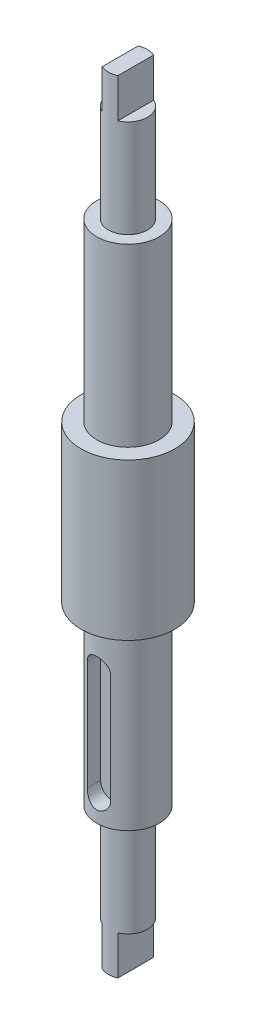
from build123d import *

# Parameters (mm, degrees)
SKETCH1_R           = 6
BOSS_EXTRUDE1_DEPTH = 10
SKETCH2_R           = 4
BOSS_EXTRUDE2_DEPTH = 22.5
SKETCH3_R           = 2.5
BOSS_EXTRUDE3_DEPTH = 12.5
BOSS_EXTRUDE4_START = 22.5
SKETCH4_R           = 4
BOSS_EXTRUDE4_DEPTH = 22.5
BOSS_EXTRUDE5_START = 12.5
SKETCH5_R           = 2.5
BOSS_EXTRUDE5_DEPTH = 12.5
BOSS_EXTRUDE6_START = 5
BOSS_EXTRUDE6_DEPTH = 5
BOSS_EXTRUDE7_DEPTH = 5
CUT_EXTRUDE1_DEPTH  = 2


with BuildPart() as part:
    # Sketch1 → Boss-Extrude1 (new, symmetric)
    with BuildSketch(Plane(origin=(0, 0, 0), x_dir=(1, 0, 0), z_dir=(0, 1, 0))):
        with Locations(Location((0, 0, 0), (0, 0, 270))):
            Circle(SKETCH1_R)
    extrude(amount=BOSS_EXTRUDE1_DEPTH, both=True)

    # Sketch2 → Boss-Extrude2 (add)
    with BuildSketch(Plane(origin=(0, 10, 0), x_dir=(1, 0, 0), z_dir=(0, 1, 0))):
        with Locations(Location((0, 0, 0), (0, 0, 90))):
            Circle(SKETCH2_R)
    extrude(amount=BOSS_EXTRUDE2_DEPTH)

    # Sketch3 → Boss-Extrude3 (add)
    with BuildSketch(Plane(origin=(0, 32.5, 0), x_dir=(1, 0, 0), z_dir=(0, 1, 0))):
        with Locations(Location((0, 0, 0), (0, 0, 270))):
            Circle(SKETCH3_R)
    extrude(amount=BOSS_EXTRUDE3_DEPTH)

    # Sketch4 → Boss-Extrude4 (add)
    with BuildSketch(Plane.XZ.offset(10).offset(BOSS_EXTRUDE4_START)):
        with Locations(Location((0, 0, 0), (0, 0, 270))):
            Circle(SKETCH4_R)
    extrude(amount=-BOSS_EXTRUDE4_DEPTH)

    # Sketch5 → Boss-Extrude5 (add)
    with BuildSketch(Plane.XZ.offset(32.5).offset(BOSS_EXTRUDE5_START)):
        with Locations(Location((0, 0, 0), (0, 0, 90))):
            Circle(SKETCH5_R)
    extrude(amount=-BOSS_EXTRUDE5_DEPTH)

    # Sketch6 → Boss-Extrude6 (add)
    with BuildSketch(Plane(origin=(0, -45, 0), x_dir=(-1, 0, 0), z_dir=(0, -1, 0)).offset(BOSS_EXTRUDE6_START)):
        with BuildLine():
            Line((1, -2.291287847), (1, 2.291287847))
            ThreePointArc((1, 2.291287847), (0, 2.5), (-1, 2.291287847))
            Line((-1, 2.291287847), (-1, -2.291287847))
            ThreePointArc((-1, -2.291287847), (0, -2.5), (1, -2.291287847))
        make_face()
    extrude(amount=-BOSS_EXTRUDE6_DEPTH)

    # Sketch7 → Boss-Extrude7 (add)
    with BuildSketch(Plane(origin=(0, 45, 0), x_dir=(1, 0, 0), z_dir=(0, 1, 0))):
        with BuildLine():
            Line((-1, 2.291287847), (-1, -2.291287847))
            ThreePointArc((-1, -2.291287847), (0, -2.5), (1, -2.291287847))
            Line((1, -2.291287847), (1, 2.291287847))
            ThreePointArc((1, 2.291287847), (0, 2.5), (-1, 2.291287847))
        make_face()
    extrude(amount=BOSS_EXTRUDE7_DEPTH)

    # Sketch8 → Cut-Extrude1 (cut)
    with BuildSketch(Plane.XY.offset(4)):
        with BuildLine():
            Line((-1.5, -29.5), (-1.5, -15.5))
            ThreePointArc((-1.5, -15.5), (0, -14), (1.5, -15.5))
            Line((1.5, -15.5), (1.5, -29.5))
            ThreePointArc((1.5, -29.5), (0, -31), (-1.5, -29.5))
        make_face()
    extrude(amount=-CUT_EXTRUDE1_DEPTH, mode=Mode.SUBTRACT)


solid = part.part
